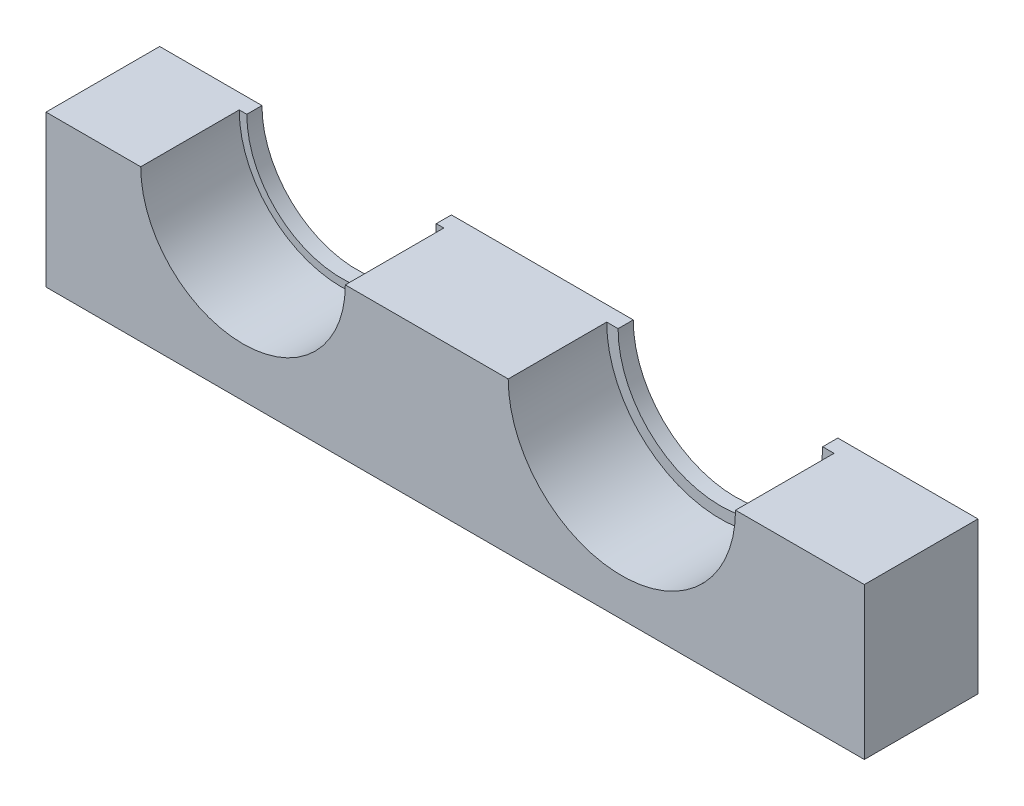
from build123d import *

# Parameters (mm, degrees)
SKETCH1_W               = 1080
SKETCH1_H               = 200
BOSS_EXTRUDE1_DEPTH     = 150
SKETCH_2_3_R            = 135
SKETCH_2_3_R_2          = 150
CUT_EXTRUDE1_DEPTH      = 130
CUT_EXTRUDE2_DEPTH      = 570.2978131
CUT_EXTRUDE2_DEPTH_BACK = 570.2978131
SKETCH_2_3_2_R          = 125
SKETCH_2_3_2_R_2        = 135


with BuildPart() as part:
    # Sketch1 → Boss-Extrude1 (new body)
    with BuildSketch(Plane.XY):
        Rectangle(SKETCH1_W, SKETCH1_H)
    extrude(amount=BOSS_EXTRUDE1_DEPTH)

    # Sketch 2_3 → Cut-Extrude1 (cut)
    with BuildSketch(Plane.XY.offset(150)):
        with Locations((-280, 100)):
            Circle(SKETCH_2_3_R)
        with Locations((220, 100)):
            Circle(SKETCH_2_3_R_2)
    extrude(amount=-CUT_EXTRUDE1_DEPTH, mode=Mode.SUBTRACT)

    # Sketch 2_3 2 → Cut-Extrude2 (cut, two sides: drawn at the far end of the back side and taken through both)
    with BuildSketch(Plane.XY.offset(150).offset(-CUT_EXTRUDE2_DEPTH_BACK)):
        with Locations((-280, 100)):
            Circle(SKETCH_2_3_2_R)
        with Locations((220, 100)):
            Circle(SKETCH_2_3_2_R_2)
    extrude(amount=CUT_EXTRUDE2_DEPTH + CUT_EXTRUDE2_DEPTH_BACK, mode=Mode.SUBTRACT)


solid = part.part
